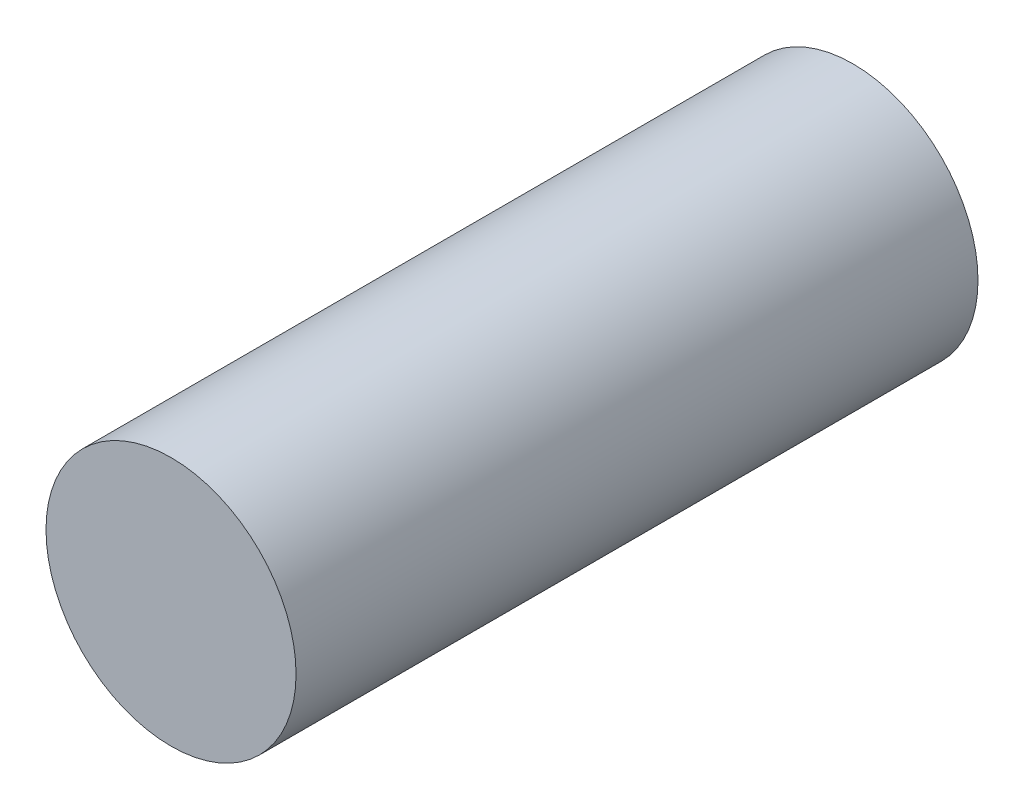
SolidWorks part; units mm, degrees
ref_plane "Front" through (0, 0, 0) normal (0, 0, 1) x (1, 0, 0)
ref_plane "Top" through (0, 0, 0) normal (0, 1, 0) x (1, 0, 0)
ref_plane "Right" through (0, 0, 0) normal (1, 0, 0) x (0, 0, -1)
sketch "Sketch1" plane through (0, 0, 0) normal (0, 0, 1) x (1, 0, 0)
  circle A0 centre (0, 0) radius 0.55
  dimension "D1" = 1.1
extrude "Boss-Extrude1" add sketch "Sketch1" along normal mid plane 3
